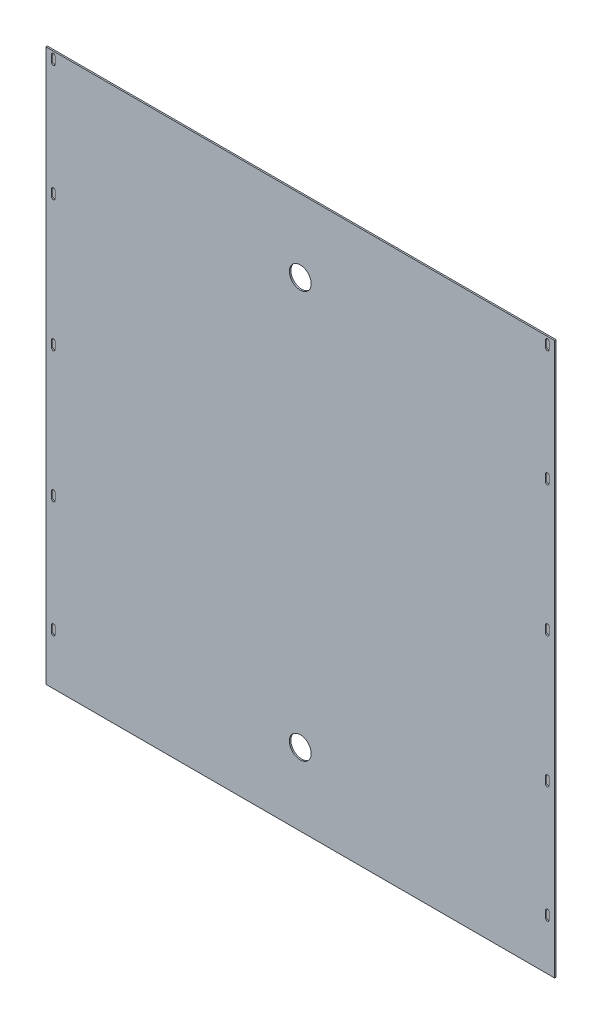
SolidWorks part; units mm, degrees
material "普通碳钢"
ref_plane "前视基准面" through (0, 0, 0) normal (0, 0, 1) x (1, 0, 0)
ref_plane "上视基准面" through (0, 0, 0) normal (0, 1, 0) x (1, 0, 0)
ref_plane "右视基准面" through (0, 0, 0) normal (1, 0, 0) x (0, 0, -1)
sketch "草图1" plane through (0, 0, 0) normal (0, 0, 1) x (1, 0, 0)
  line L1 (-350, 380) -> (350, 380)
  line L2 (-350, 380) -> (-350, -380)
  line L3 (-350, -380) -> (350, -380)
  line L4 (350, 380) -> (350, -380)
  line L5 (0, -380) -> (0, 380) construction
  line L6 (-350, 0) -> (350, 0) construction
  point P0 (0, 0)
  dimension "D1" = 700
  dimension "D2" = 760
extrude "凸台-拉伸1" add sketch "草图1" along normal blind 2
sketch "草图2" plane through (0, 0, 2) normal (0, 0, 1) x (1, 0, 0)
  line L0 (-340, 210) -> (340, 210) construction
  line L1 (-340, -310) -> (340, -310) construction
  line L2 (-340, -310) -> (-340, 370) construction
  line L3 (-340, 370) -> (340, 370) construction
  line L4 (340, -310) -> (340, 370) construction
  line L5 (0, 370) -> (0, -310) construction
  line L6 (-350, -380) -> (350, -380) construction
  line L7 (-340, -150) -> (340, -150) construction
  line L8 (-340, 375) -> (-340, 365) construction
  line L9 (-337.75, 375) -> (-337.75, 365)
  line L10 (-342.25, 375) -> (-342.25, 365)
  line L11 (-340, 205) -> (-340, 215) construction
  line L12 (-342.25, 205) -> (-342.25, 215)
  line L13 (-337.75, 205) -> (-337.75, 215)
  line L14 (-340, 25) -> (-340, 35) construction
  line L15 (-342.25, 25) -> (-342.25, 35)
  line L16 (-337.75, 25) -> (-337.75, 35)
  line L17 (340, 375) -> (340, 365) construction
  line L18 (337.75, 375) -> (337.75, 365)
  line L19 (342.25, 375) -> (342.25, 365)
  line L20 (340, 205) -> (340, 215) construction
  line L21 (342.25, 205) -> (342.25, 215)
  line L22 (337.75, 205) -> (337.75, 215)
  line L23 (340, 25) -> (340, 35) construction
  line L24 (342.25, 25) -> (342.25, 35)
  line L25 (337.75, 25) -> (337.75, 35)
  line L26 (-340, -315) -> (-340, -305) construction
  line L27 (-337.75, -315) -> (-337.75, -305)
  line L28 (-342.25, -315) -> (-342.25, -305)
  line L29 (-340, -155) -> (-340, -145) construction
  line L30 (-337.75, -155) -> (-337.75, -145)
  line L31 (-342.25, -155) -> (-342.25, -145)
  line L32 (340, -315) -> (340, -305) construction
  line L33 (337.75, -315) -> (337.75, -305)
  line L34 (342.25, -315) -> (342.25, -305)
  line L35 (340, -145) -> (340, -155) construction
  line L36 (342.25, -145) -> (342.25, -155)
  line L37 (337.75, -145) -> (337.75, -155)
  line L38 (-340, -310) -> (340, -310) construction
  line L39 (-340, -150) -> (340, -150) construction
  arc A0 (-337.75, 375) -> (-342.25, 375) centre (-340, 375) ccw
  arc A1 (-342.25, 365) -> (-337.75, 365) centre (-340, 365) ccw
  arc A2 (-342.25, 205) -> (-337.75, 205) centre (-340, 205) ccw
  arc A3 (-337.75, 215) -> (-342.25, 215) centre (-340, 215) ccw
  arc A4 (-342.25, 25) -> (-337.75, 25) centre (-340, 25) ccw
  arc A5 (-337.75, 35) -> (-342.25, 35) centre (-340, 35) ccw
  arc A6 (337.75, 375) -> (342.25, 375) centre (340, 375) cw
  arc A7 (342.25, 365) -> (337.75, 365) centre (340, 365) cw
  arc A8 (342.25, 205) -> (337.75, 205) centre (340, 205) cw
  arc A9 (337.75, 215) -> (342.25, 215) centre (340, 215) cw
  arc A10 (342.25, 25) -> (337.75, 25) centre (340, 25) cw
  arc A11 (337.75, 35) -> (342.25, 35) centre (340, 35) cw
  arc A12 (-337.75, -315) -> (-342.25, -315) centre (-340, -315) cw
  arc A13 (-342.25, -305) -> (-337.75, -305) centre (-340, -305) cw
  arc A14 (-337.75, -155) -> (-342.25, -155) centre (-340, -155) cw
  arc A15 (-342.25, -145) -> (-337.75, -145) centre (-340, -145) cw
  arc A16 (337.75, -315) -> (342.25, -315) centre (340, -315) ccw
  arc A17 (342.25, -305) -> (337.75, -305) centre (340, -305) ccw
  arc A18 (342.25, -145) -> (337.75, -145) centre (340, -145) ccw
  arc A19 (337.75, -155) -> (342.25, -155) centre (340, -155) ccw
  point P0 (0, 0)
  point P9 (-340, 210)
  point P10 (-340, 370)
  point P11 (-340, 30)
  point P12 (-340, -150)
  point P13 (-340, -310)
  point P14 (340, -310)
  point P15 (340, -150)
  point P16 (340, 0)
  point P17 (340, 210)
  point P18 (340, 370)
  point P20 (-340, 370)
  point P27 (-340, 210)
  point P34 (-340, 30)
  point P41 (340, 370)
  point P48 (340, 210)
  point P55 (340, 30)
  point P62 (-340, -310)
  point P69 (-340, -150)
  point P76 (340, -310)
  point P83 (340, -150)
  dimension "D1" = 680
  dimension "D2" = 680
  dimension "D3" = 360
  dimension "D4" = 10
  dimension "D5" = 4.5
  dimension "D6" = 10
  dimension "D7" = 4.5
  dimension "D8" = 4.5
  dimension "D9" = 10
  dimension "D10" = 70
  dimension "D11" = 160
extrude "切除-拉伸1" cut sketch "草图2" against normal blind 10
sketch "草图3" plane through (0, 0, 2) normal (0, 0, 1) x (1, 0, 0)
  line L0 (0, 0) -> (490.012, 0) construction
  line L1 (-350, -380) -> (350, -380) construction
  circle A0 centre (0, -280) radius 15
  circle A1 centre (0, 280) radius 15
  point P4 (0, 0)
  dimension "D2" = 30
  dimension "D1" = 100
extrude "切除-拉伸2" cut sketch "草图3" against normal blind 10
